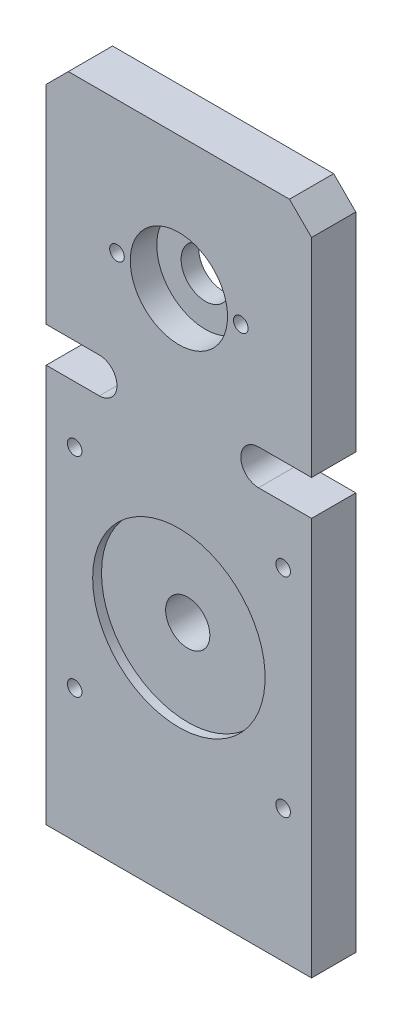
SolidWorks part; units mm, degrees
ref_plane "Front Plane" through (0, 0, 0) normal (0, 0, 1) x (1, 0, 0)
ref_plane "Top Plane" through (0, 0, 0) normal (0, 1, 0) x (1, 0, 0)
ref_plane "Right Plane" through (0, 0, 0) normal (1, 0, 0) x (0, 0, -1)
sketch "Sketch1" plane through (0, 0, 0) normal (0, 0, 1) x (1, 0, 0)
  line L1 (-30, 75) -> (30, 75)
  line L2 (-30, 75) -> (-30, -75)
  line L3 (-30, -75) -> (30, -75)
  line L4 (30, 75) -> (30, -75)
  line L5 (-30, 75) -> (30, -75) construction
  line L6 (-30, -75) -> (30, 75) construction
  point P0 (0, 0)
  dimension "D1" = 60
  dimension "D2" = 150
extrude "Boss-Extrude1" add sketch "Sketch1" along normal blind 10
chamfer "Chamfer1" distance 5 angle 45 2 edges at (30, 75, 5) (-30, 75, 5)
sketch "Sketch5" plane through (0, 0, 0) normal (0, 0, -1) x (-1, 0, 0)
  circle A0 centre (0, -21.425) radius 19.5
  dimension "D1" = 39
extrude "Cut-Extrude5" cut sketch "Sketch5" along normal blind 2 from offset 10 offset against normal yes
sketch "Sketch6" plane through (0, 0, 8) normal (0, 0, 1) x (1, 0, 0)
  circle A0 centre (0, -21.425) radius 5
  dimension "D1" = 10
extrude "Cut-Extrude6" cut sketch "Sketch6" against normal through all
hole_wizard "M4 Tapped Hole1" positions "Sketch8" profile "Sketch7" tap size "M4" standard "GB" end condition through all
sketch "Sketch8" plane through (0, 0, 10) normal (0, 0, 1) x (1, 0, 0)
  point P1 (-23.57, 2.145)
  point P5 (-23.57, -44.995)
  point P9 (23.57, 2.145)
  point P13 (23.57, -44.995)
sketch "Sketch7" plane through (-23.57, 2.145, 10) normal (1, 0, 0) x (0, -1, 0)
  line L0 (0, 0) -> (0, 10)
  line L1 (0, 10) -> (1.65, 10)
  line L2 (1.65, 10) -> (1.65, 0)
  line L5 (1.65, 0) -> (0, 0)
  line L11 (0, -6.35) -> (0, 107.95) construction
  dimension "通孔螺纹孔钻头直径" = 3.3
  dimension "通孔螺纹孔钻头深度" = 10
cosmetic thread "Cosmetic Thread 1" parameters "D2"=4
cosmetic thread "Cosmetic Thread 2" parameters "D2"=4
cosmetic thread "Cosmetic Thread 3" parameters "D2"=4
cosmetic thread "Cosmetic Thread 4" parameters "D2"=4
sketch "Sketch9" plane through (0, 0, 10) normal (0, 0, 1) x (1, 0, 0)
  line L0 (0, 75) -> (0, -75) construction
  line L1 (25, 75) -> (-25, 75) construction
  line L2 (-30, -75) -> (30, -75) construction
  circle A0 centre (0, 45) radius 11
  dimension "D2" = 22
  dimension "D1" = 30
extrude "Cut-Extrude7" cut sketch "Sketch9" against normal blind 6
sketch "Sketch10" plane through (0, 0, 4) normal (0, 0, 1) x (1, 0, 0)
  circle A0 centre (0, 45) radius 5.5
  circle A1 centre (0, 45) radius 11 construction
  dimension "D1" = 11
extrude "Cut-Extrude8" cut sketch "Sketch10" against normal through all
sketch "Sketch11" plane through (0, 0, 0) normal (0, 0, -1) x (-1, 0, 0)
  line L0 (18, 19) -> (40.9927, 19) construction
  line L1 (18, 23) -> (40.9927, 23)
  line L2 (18, 15) -> (40.9927, 15)
  line L3 (-30, -83) -> (30, -83) construction
  line L4 (30, 70) -> (30, -75) construction
  arc A0 (18, 23) -> (18, 15) centre (18, 19) ccw
  arc A1 (40.9927, 15) -> (40.9927, 23) centre (40.9927, 19) ccw
  point P2 (29.4964, 19)
  dimension "D1" = 8
  dimension "D2" = 102
  dimension "D3" = 12
extrude "Cut-Extrude9" cut sketch "Sketch11" against normal through all
mirror "Mirror1" about plane through (0, 0, 0) normal (1, 0, 0) of "Cut-Extrude9"
hole_wizard "M4 Tapped Hole2" positions "Sketch12" profile "Sketch13" tap size "M4" standard "GB" end condition through all
sketch "Sketch12" plane through (0, 0, 10) normal (0, 0, 1) x (1, 0, 0)
  line L0 (0, 45) -> (-39.3261, 45) construction
  line L2 (0, 45) -> (0, 81.9465) construction
  point P0 (-14, 45)
  point P17 (14, 45)
  dimension "D1" = 14
sketch "Sketch13" plane through (-14, 45, 10) normal (1, 0, 0) x (0, -1, 0)
  line L0 (0, 0) -> (0, 10)
  line L1 (0, 10) -> (1.65, 10)
  line L2 (1.65, 10) -> (1.65, 0)
  line L5 (1.65, 0) -> (0, 0)
  line L11 (0, -6.35) -> (0, 107.95) construction
  dimension "通孔螺纹孔钻头直径" = 3.3
  dimension "通孔螺纹孔钻头深度" = 10
cosmetic thread "Cosmetic Thread 5" parameters "D2"=4
cosmetic thread "Cosmetic Thread 6" parameters "D2"=4
hole_wizard "M4 Tapped Hole3" positions "Sketch15" profile "Sketch14" tap size "M4" standard "GB"
sketch "Sketch15" plane through (0, -75, 0) normal (0, -1, 0) x (-1, 0, 0)
  line L1 (20, -5) -> (-20, -5) construction
  line L2 (30, -10) -> (-30, -10) construction
  line L3 (30, 0) -> (-30, 0) construction
  line L4 (-30, -10) -> (-30, 0) construction
  line L5 (0, 0) -> (0, -5) construction
  point P9 (-20, -5)
  point P10 (20, -5)
  dimension "D1" = 10
sketch "Sketch14" plane through (-20, -75, 5) normal (1, 0, 0) x (0, 0, -1)
  line L0 (0, 0) -> (0, 12.4914)
  line L1 (0, 12.4914) -> (1.65, 11.5)
  line L2 (1.65, 11.5) -> (1.65, 0)
  line L5 (1.65, 0) -> (0, 0)
  line L10 (0, 12.4914) -> (-1.65, 11.5) construction
  line L11 (0, -6.35) -> (0, 107.95) construction
  dimension "螺纹孔钻头直径" = 3.3
  dimension "螺纹孔钻头深度" = 11.5
  dimension "导头角度" = 118
cosmetic thread "Cosmetic Thread 7" parameters "D1"=8, "D2"=4
cosmetic thread "Cosmetic Thread 8" parameters "D1"=8, "D2"=4
